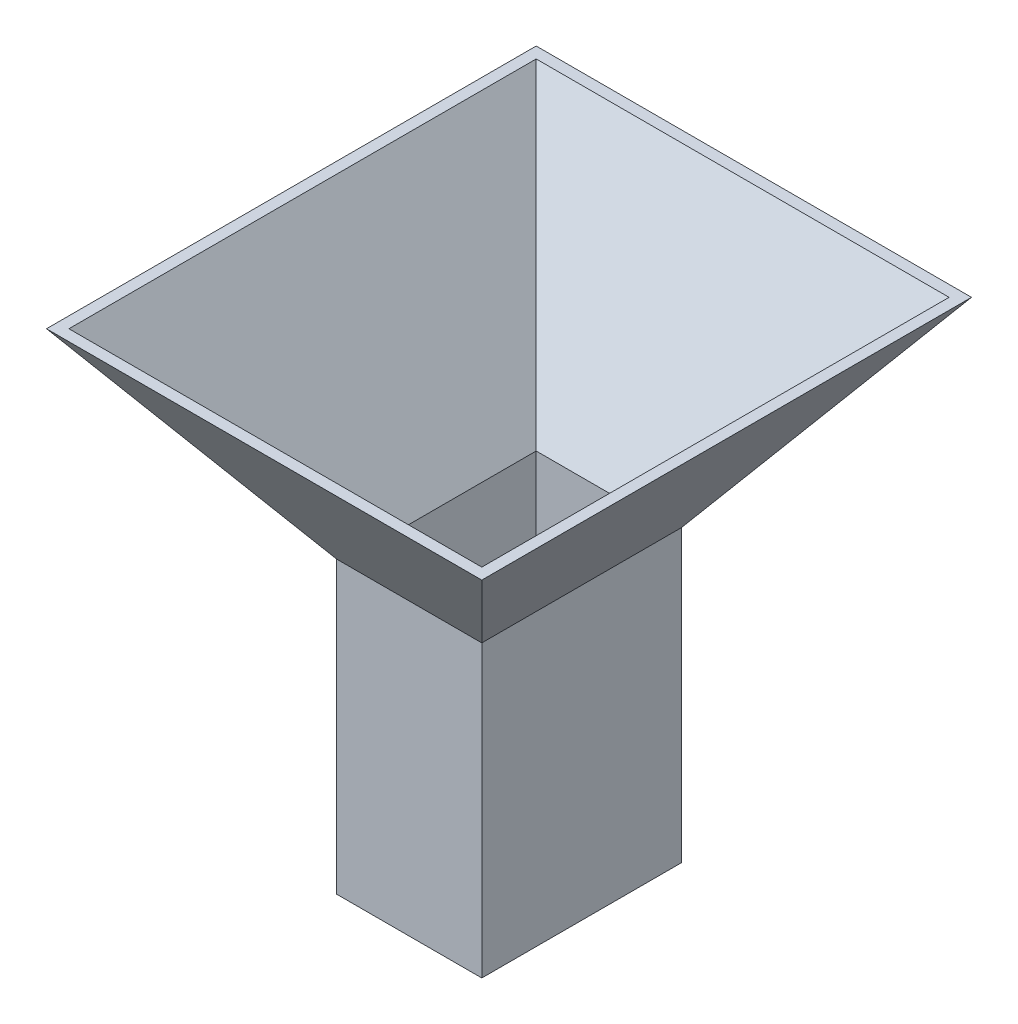
from build123d import *

# Parameters (mm, degrees)
SKETCH_1_W          = 80
SKETCH_1_H          = 110
EXTRUDE_1_DEPTH     = 160
SHELL_1_T           = -5
SKETCH_7_W          = 62
SKETCH_7_H          = 20
CUT_EXTRUDE_3_DEPTH = 5


with BuildPart() as part:
    # 草图1 → 凸台-拉伸1 (new body)
    with BuildSketch(Plane(origin=(0, 0, 0), x_dir=(1, 0, 0), z_dir=(0, 1, 0))):
        Rectangle(SKETCH_1_W, SKETCH_1_H)
    extrude(amount=EXTRUDE_1_DEPTH)

    # 草图3 → 放样1 section 0
    with BuildSketch(Plane(origin=(0, 270, 0), x_dir=(1, 0, 0), z_dir=(0, 1, 0))):
        with BuildLine():
            Line((-120, -135), (120, -135))
            Line((120, -135), (120, 135))
            Line((120, 135), (-120, 135))
            Line((-120, 135), (-120, -135))
        make_face()
    # 草图2 → 放样1 section 1
    with BuildSketch(Plane(origin=(0, 160, 0), x_dir=(1, 0, 0), z_dir=(0, 1, 0))):
        with BuildLine():
            Line((40, -55), (40, 55))
            Line((40, 55), (-40, 55))
            Line((-40, 55), (-40, -55))
            Line((-40, -55), (40, -55))
        make_face()
    loft()

    # 抽壳1
    shell_1_openings = [part.faces().sort_by_distance(p)[0] for p in [
        (0, 270, 0),
        (0, 0, 0),
    ]]
    offset(amount=SHELL_1_T, openings=shell_1_openings, kind=Kind.INTERSECTION)

    # 草图7 → 切除-拉伸3 (cut)
    with BuildSketch(Plane(origin=(0, 0, -55), x_dir=(-1, 0, 0), z_dir=(0, 0, -1))):
        with Locations((0, 55)):
            Rectangle(SKETCH_7_W, SKETCH_7_H)
    extrude(amount=-CUT_EXTRUDE_3_DEPTH, mode=Mode.SUBTRACT)


solid = part.part
